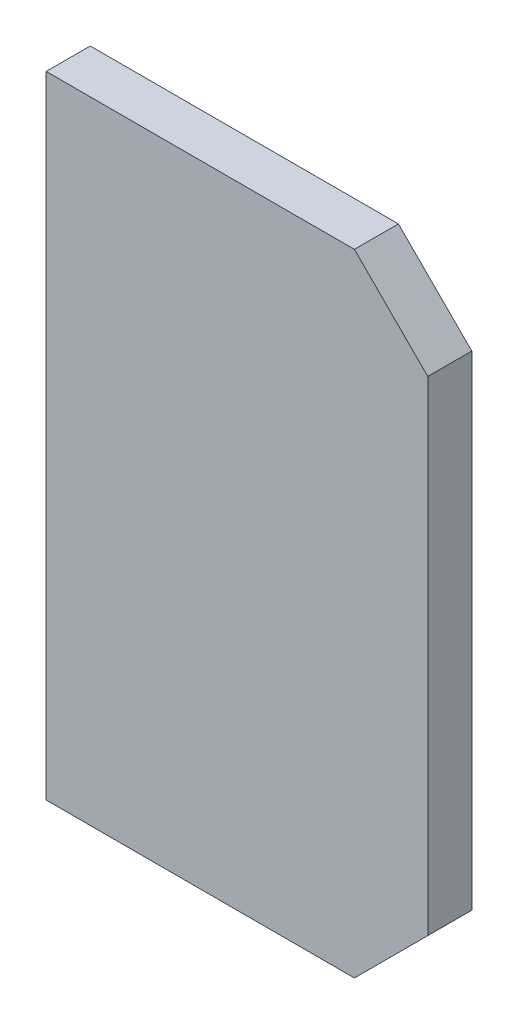
from build123d import *

# Parameters (mm, degrees)
SKETCH_1_W      = 26
SKETCH_1_H      = 43
EXTRUDE_1_DEPTH = 3
CHAMFER_1_SIZE  = 5


with BuildPart() as part:
    # 草图1 → 凸台-拉伸1 (new body)
    with BuildSketch(Plane.XY):
        with Locations((13, 21.5)):
            Rectangle(SKETCH_1_W, SKETCH_1_H)
    extrude(amount=EXTRUDE_1_DEPTH)

    # 倒角1
    chamfer_1_edges = [part.edges().sort_by_distance(p)[0] for p in [
        (26, 43, 1.5),
        (26, 0, 1.5),
    ]]
    chamfer(chamfer_1_edges, length=CHAMFER_1_SIZE)


solid = part.part
